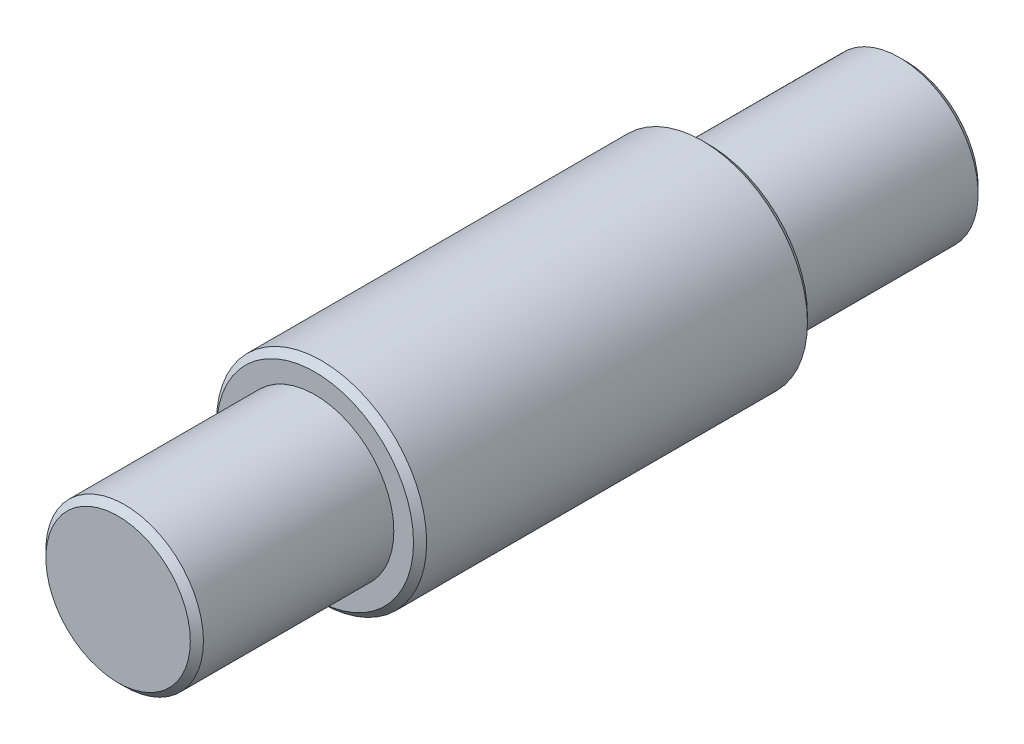
SolidWorks part; units mm, degrees
ref_plane "Front Plane" through (0, 0, 0) normal (0, 0, 1) x (1, 0, 0)
ref_plane "Top Plane" through (0, 0, 0) normal (0, 1, 0) x (1, 0, 0)
ref_plane "Right Plane" through (0, 0, 0) normal (1, 0, 0) x (0, 0, -1)
sketch "Sketch1" plane through (0, 0, 0) normal (0, 0, 1) x (1, 0, 0)
  circle A0 centre (0, 0) radius 6
extrude "Boss-Extrude1" add sketch "Sketch1" along normal blind 15
sketch "Sketch2" plane through (0, 0, 0) normal (0, 0, -1) x (-1, 0, 0)
  circle A0 centre (0, 0) radius 8
extrude "Boss-Extrude2" add sketch "Sketch2" along normal blind 30 contours A0
sketch "Sketch3" plane through (0, 0, -30) normal (0, 0, -1) x (-1, 0, 0)
  circle A0 centre (0, 0) radius 6
extrude "Boss-Extrude3" add sketch "Sketch3" along normal blind 15
chamfer "Chamfer1" distance 0.5 angle 45 4 edges at (6, 0, 15) (-6, 0, -45) (-8, 0, -30) (-8, 0, 0)
